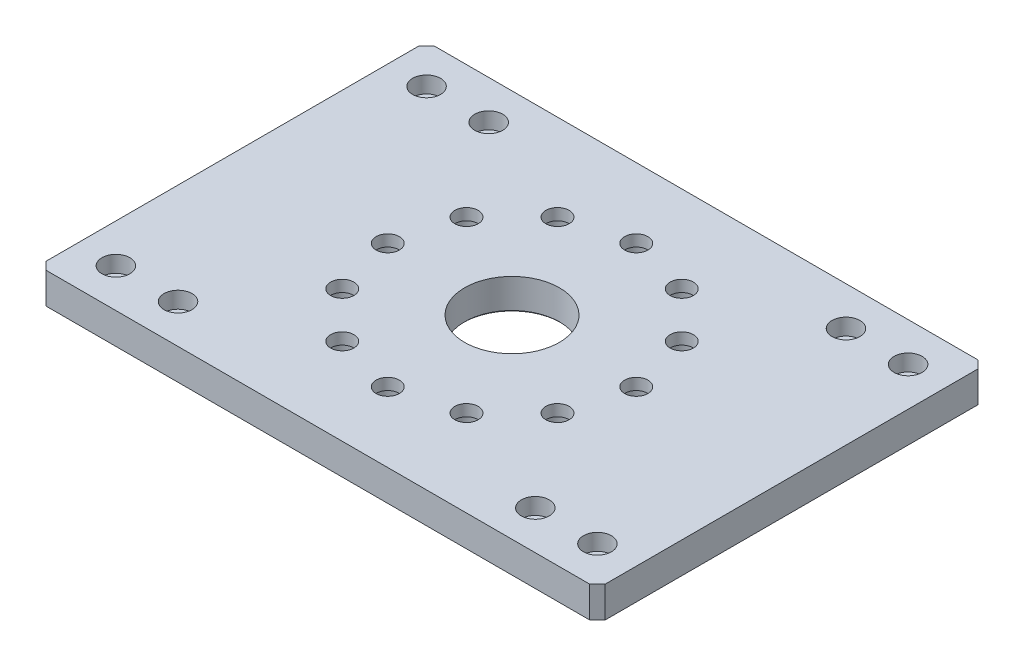
from build123d import *

# Parameters (mm, degrees)
SKETCH_1_W                    = 360
SKETCH_1_H                    = 250
EXTRUDE_1_DEPTH               = 20
HOLE_WIZARD_M10_1_D           = 12
HOLE_WIZARD_M10_1_CBORE_D     = 18
HOLE_WIZARD_M10_1_CBORE_DEPTH = 10.6
HOLE_WIZARD_M52_1_D           = 61
HOLE_WIZARD_M12_1_D           = 15
HOLE_WIZARD_M12_1_CBORE_D     = 20
HOLE_WIZARD_M12_1_CBORE_DEPTH = 12.6
CHAMFER_1_SIZE                = 1
CHAMFER_2_SIZE                = 5


with BuildPart() as part:
    # 草图1 → 凸台-拉伸1 (new body)
    with BuildSketch(Plane.XZ.offset(-63)):
        with Locations((315.1, -245)):
            Rectangle(SKETCH_1_W, SKETCH_1_H)
    extrude(amount=-EXTRUDE_1_DEPTH)

    # M10 六角凹头螺钉的柱形沉头孔1 (through all)
    with Locations(Plane(origin=(0, 83, 0), x_dir=(-1, 0, 0), z_dir=(0, 1, 0))):
        with Locations((-470.1, -345), (-430.1, -345), (-470.1, -145), (-430.1, -145), (-200.1, -145), (-200.1, -345), (-160.1, -145), (-160.1, -345)):
            CounterBoreHole(HOLE_WIZARD_M10_1_D / 2, HOLE_WIZARD_M10_1_CBORE_D / 2, HOLE_WIZARD_M10_1_CBORE_DEPTH)

    # M52 间隙孔1 (through all)
    with Locations(Plane(origin=(0, 63, 0), x_dir=(-1, 0, 0), z_dir=(0, -1, 0))):
        with Locations((-315.1, 245)):
            Hole(HOLE_WIZARD_M52_1_D / 2)

    # M12 六角凹头螺钉的柱形沉头孔1 (through all)
    with Locations(Plane(origin=(0, 63, 0), x_dir=(-1, 0, 0), z_dir=(0, -1, 0))):
        with Locations((-245.817967697, 205), (-275.1, 175.717967697), (-315.1, 165), (-355.1, 175.717967697), (-384.382032303, 205), (-395.1, 245), (-384.382032303, 285), (-355.1, 314.282032303), (-315.1, 325), (-275.1, 314.282032303), (-245.817967697, 285), (-235.1, 245)):
            CounterBoreHole(HOLE_WIZARD_M12_1_D / 2, HOLE_WIZARD_M12_1_CBORE_D / 2, HOLE_WIZARD_M12_1_CBORE_DEPTH)

    # 倒角1
    chamfer_1_edges = [part.edges().sort_by_distance(p)[0] for p in [
        (284.6, 63, -245),
    ]]
    chamfer(chamfer_1_edges, length=CHAMFER_1_SIZE)

    # 倒角2
    chamfer_2_edges = [part.edges().sort_by_distance(p)[0] for p in [
        (495.1, 73, -120),
        (495.1, 73, -370),
        (135.1, 73, -370),
        (135.1, 73, -120),
    ]]
    chamfer(chamfer_2_edges, length=CHAMFER_2_SIZE)


solid = part.part
